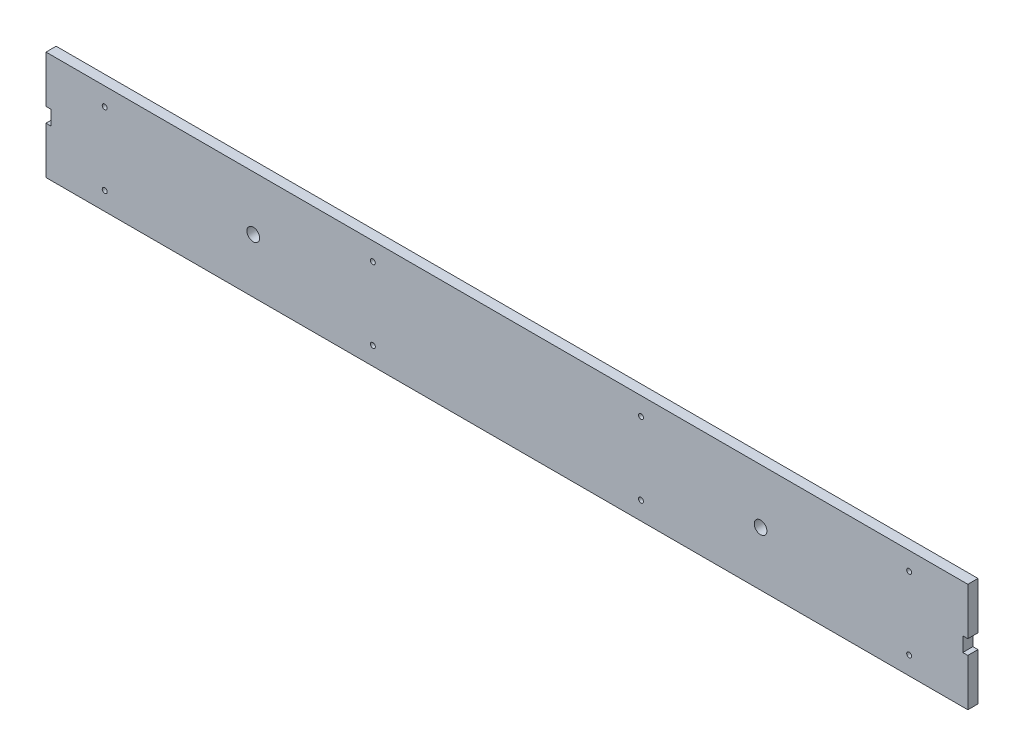
from build123d import *

# Parameters (mm, degrees)
SKETCH1_W           = 1272
SKETCH1_H           = 150
SKETCH1_R           = 8.75
BOSS_EXTRUDE1_DEPTH = 14
M8_TAPPED_HOLE1_D   = 6.8
SKETCH5_W           = 14
SKETCH5_H           = 20
CUT_EXTRUDE1_DEPTH  = 1281.890315367


with BuildPart() as part:
    # Sketch1 → Boss-Extrude1 (new body)
    with BuildSketch(Plane.XY):
        with Locations((636, 75)):
            Rectangle(SKETCH1_W, SKETCH1_H)
        with Locations((286, 75)):
            Circle(SKETCH1_R, mode=Mode.SUBTRACT)
        with Locations((986, 75)):
            Circle(SKETCH1_R, mode=Mode.SUBTRACT)
    extrude(amount=BOSS_EXTRUDE1_DEPTH)

    # M8 Tapped Hole1 (through all)
    with Locations(Plane(origin=(81, 125, 14), x_dir=(1, 0, 0), z_dir=(0, 0, 1))):
        with Locations((0, 0), (0, -100), (370, 0), (370, -100), (740, 0), (740, -100), (1110, 0), (1110, -100)):
            Hole(M8_TAPPED_HOLE1_D / 2)

    # Sketch5 → Cut-Extrude1 (cut, through all)
    with BuildSketch(Plane.XY.offset(14)):
        with Locations((0, 75)):
            Rectangle(SKETCH5_W, SKETCH5_H)
        with Locations((1272, 75)):
            Rectangle(SKETCH5_W, SKETCH5_H)
    extrude(amount=-CUT_EXTRUDE1_DEPTH, mode=Mode.SUBTRACT)


solid = part.part
